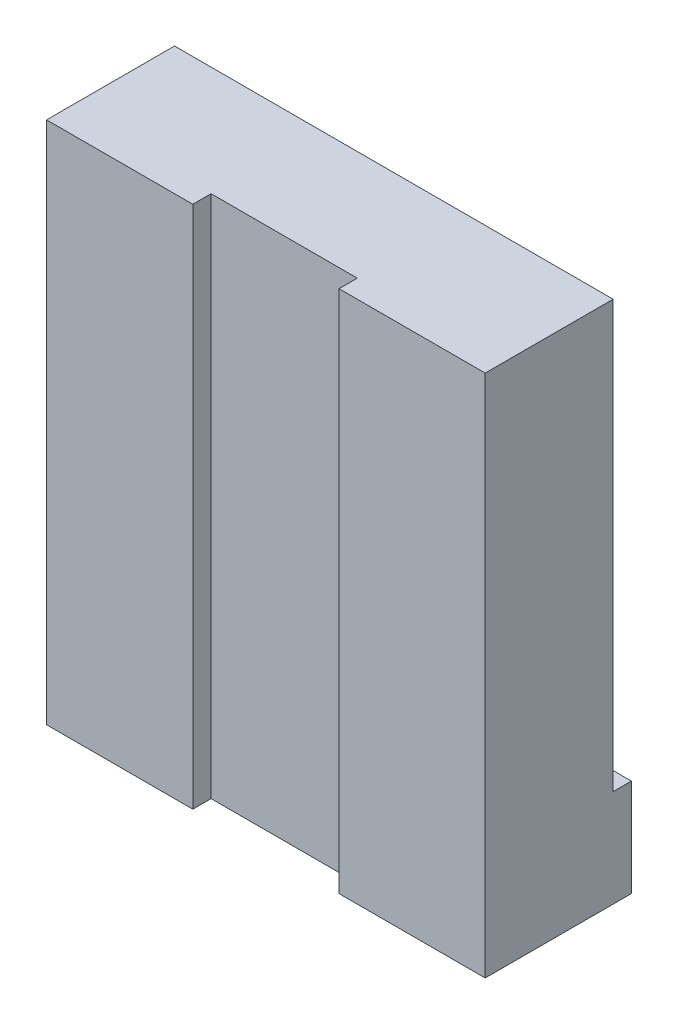
SolidWorks part; units mm, degrees
ref_plane "前视基准面" through (0, 0, 0) normal (0, 0, 1) x (1, 0, 0)
ref_plane "上视基准面" through (0, 0, 0) normal (0, 1, 0) x (1, 0, 0)
ref_plane "右视基准面" through (0, 0, 0) normal (1, 0, 0) x (0, 0, -1)
sketch "草图1" plane through (0, 0, 0) normal (0, 0, 1) x (1, 0, 0)
  line L1 (-18, -21.5) -> (18, -21.5)
  line L2 (-18, -21.5) -> (-18, 21.5)
  line L3 (-18, 21.5) -> (18, 21.5)
  line L4 (18, -21.5) -> (18, 21.5)
  line L5 (-18, -21.5) -> (18, 21.5) construction
  line L6 (-18, 21.5) -> (18, -21.5) construction
  point P0 (0, 0)
  dimension "D1" = 43
  dimension "D2" = 36
extrude "凸台-拉伸1" add sketch "草图1" along normal mid plane 12
sketch "草图2" plane through (0, 0, 6) normal (0, 0, 1) x (1, 0, 0)
  line L0 (-18, -21.5) -> (18, -21.5) construction
  line L1 (6, 21.5) -> (-6, 21.5)
  line L2 (6, 21.5) -> (6, -21.5)
  line L3 (6, -21.5) -> (-6, -21.5)
  line L4 (-6, 21.5) -> (-6, -21.5)
  line L5 (0, 0) -> (0, 21.5) construction
  line L6 (18, 21.5) -> (-18, 21.5) construction
  point P7 (6, 30)
  dimension "D1" = 12
extrude "切除-拉伸1" cut sketch "草图2" against normal blind 1.5
sketch "草图3" plane through (0, 0, -6) normal (0, 0, -1) x (-1, 0, 0)
  line L0 (18, -21.5) -> (-18, -21.5) construction
  line L1 (15.25, 21.5) -> (-15.25, 21.5)
  line L2 (15.25, 21.5) -> (15.25, -21.5)
  line L3 (15.25, -21.5) -> (-15.25, -21.5)
  line L4 (-15.25, 21.5) -> (-15.25, -21.5)
  line L5 (15.25, 21.5) -> (-15.25, -21.5) construction
  line L6 (15.25, -21.5) -> (-15.25, 21.5) construction
  point P0 (0, 0)
  dimension "D1" = 30.5
extrude "切除-拉伸2" cut sketch "草图3" against normal blind 1.5
sketch "草图4" plane through (0, 0, -6) normal (0, 0, -1) x (-1, 0, 0)
  line L0 (-18, -21.5) -> (-18, 21.5) construction
  line L1 (18, 21.5) -> (-18, 21.5)
  line L2 (18, 21.5) -> (18, -13.5)
  line L3 (18, -13.5) -> (-18, -13.5)
  line L4 (-18, 21.5) -> (-18, -13.5)
  dimension "D1" = 35
extrude "切除-拉伸3" cut sketch "草图4" against normal blind 1.5
